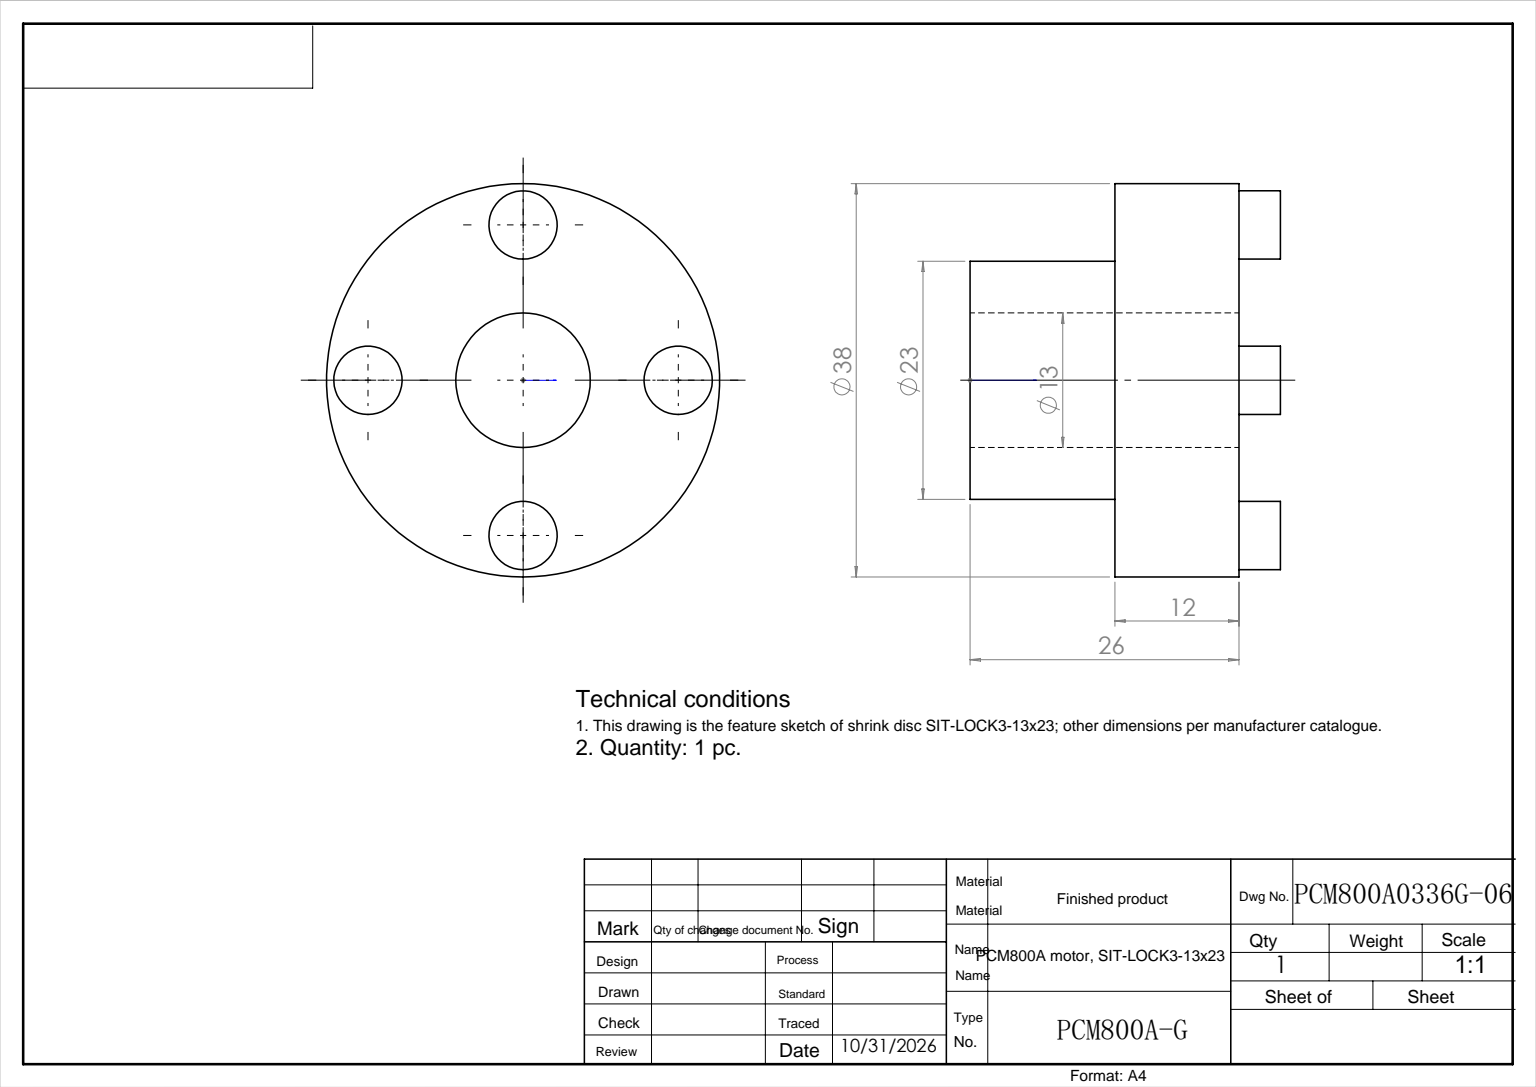
from build123d import *

# Parameters (mm, degrees)
SKETCH_1_R      = 11.5
SKETCH_1_R_2    = 6.5
EXTRUDE_1_DEPTH = 14
SKETCH_2_R      = 19
SKETCH_2_R_2    = 6.5
EXTRUDE_2_DEPTH = 12
SKETCH_3_R      = 3.3
EXTRUDE_3_DEPTH = 4


with BuildPart() as part:
    # 草图1 → 拉伸1 (new body)
    with BuildSketch(Plane(origin=(0, 0, 0), x_dir=(1, 0, 0), z_dir=(0, 1, 0))):
        with Locations(Location((0, 0, 0), (0, 0, 270))):
            Circle(SKETCH_1_R)
        with Locations(Location((0, 0, 0), (0, 0, 270))):
            Circle(SKETCH_1_R_2, mode=Mode.SUBTRACT)
    extrude(amount=EXTRUDE_1_DEPTH)

    # 草图2 → 拉伸2 (add)
    with BuildSketch(Plane(origin=(0, 14, 0), x_dir=(-1, 0, 0), z_dir=(0, 1, 0))):
        with Locations(Location((0, 0, 0), (0, 0, 90))):
            Circle(SKETCH_2_R)
        with Locations(Location((0, 0, 0), (0, 0, 90))):
            Circle(SKETCH_2_R_2, mode=Mode.SUBTRACT)
    extrude(amount=EXTRUDE_2_DEPTH)

    # 草图3 → 拉伸3 (add)
    with BuildSketch(Plane(origin=(0, 26, 0), x_dir=(-1, 0, 0), z_dir=(0, 1, 0))):
        with Locations(Location((-15, 0, 0), (0, 0, 90))):
            Circle(SKETCH_3_R)
        with Locations(Location((0, -15, 0), (0, 0, 90))):
            Circle(SKETCH_3_R)
        with Locations(Location((0, 15, 0), (0, 0, 90))):
            Circle(SKETCH_3_R)
        with Locations(Location((15, 0, 0), (0, 0, 90))):
            Circle(SKETCH_3_R)
    extrude(amount=EXTRUDE_3_DEPTH)


solid = part.part
